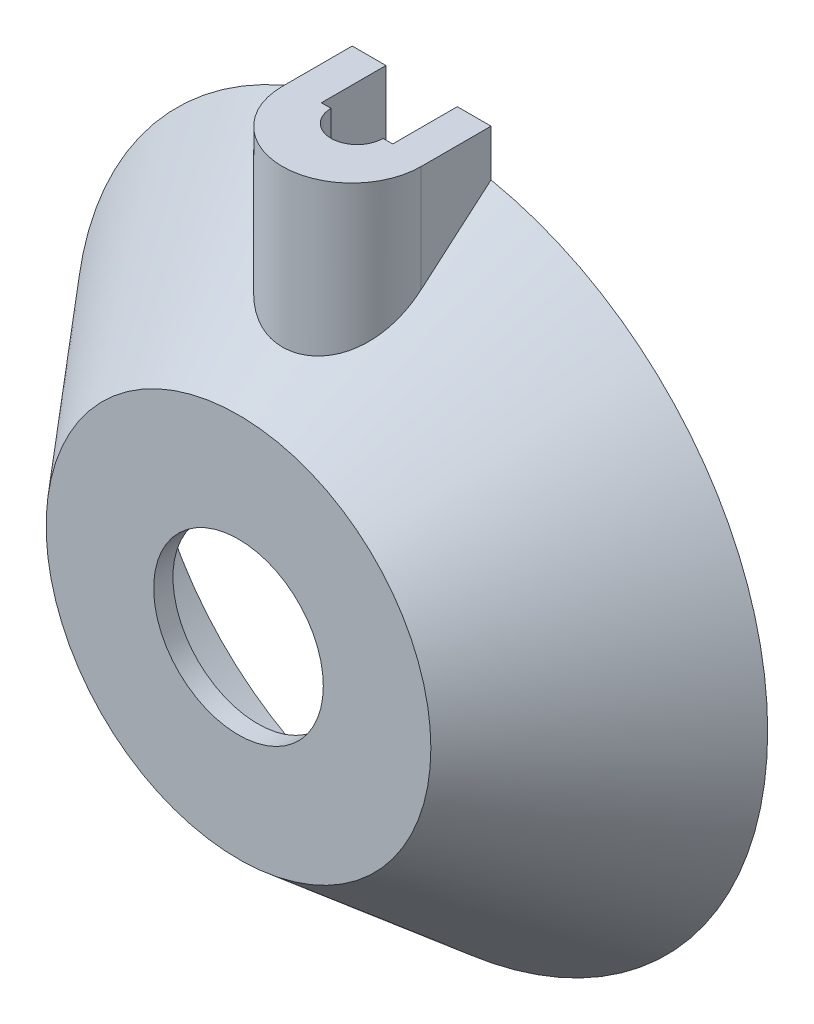
from build123d import *

# Parameters (mm, degrees)
SKETCH_1_R           = 35.9
EXTRUDE_1_DEPTH      = 19
EXTRUDE_1_TAPER      = 40
EXTRUDE_2_DEPTH      = 40
EXTRUDE_3_REACH      = 59.007
SKETCH_8_R           = 31
SKETCH_8_R_2         = 29
SKETCH_9_R           = 8.8
CUT_EXTRUDE_1_DEPTH  = 2
CUT_EXTRUDE_2_DEPTH  = 16
EXTRUDE_4_REACH      = 88.085
EXTRUDE_4_END_RADIUS = 31
SKETCH_11_W          = 2.2
SKETCH_11_H          = 6.7


with BuildPart() as part:
    # 草图1 → 凸台-拉伸1 (new body)
    with BuildSketch(Plane.XY):
        Circle(SKETCH_1_R)
    extrude(amount=EXTRUDE_1_DEPTH, taper=EXTRUDE_1_TAPER)

    # 草图6 → 凸台-拉伸2 (add)
    with BuildSketch(Plane(origin=(0, 0, 0), x_dir=(1, 0, 0), z_dir=(0, 1, 0))):
        with BuildLine():
            Line((-7.2, 0), (-7.2, -7.25))
            ThreePointArc((-7.2, -7.25), (0, -14.45), (7.2, -7.25))
            Line((7.2, -7.25), (7.2, 0))
            Line((7.2, 0), (-7.2, 0))
        make_face()
    extrude(amount=EXTRUDE_2_DEPTH)

    # 草图7 → 切除-旋转1 (revolve, cut)
    with BuildSketch(Plane(origin=(0, 0, 0), x_dir=(0, 0, -1), z_dir=(1, 0, 0)), mode=Mode.PRIVATE) as cut_revolve_1_sk:
        Polygon((-17, 0), (-17, -17.63530627), (0, -31.9), (0, 0), align=None)
    revolve(cut_revolve_1_sk.sketch.rotate(Axis((0, 0, -9.48864884), (0, 0, 1)), 270), axis=Axis((0, 0, -9.48864884), (0, 0, 1)), mode=Mode.SUBTRACT)

    # 凸台-拉伸3: up to this cone (the profile starts inside it)
    extrude_3_end = Plane(origin=(0, 0, 0), z_dir=(0, 0, -1)).offset(-38.016938604) * Cone(1e-06, 108.599579987, 129.423938604, align=(Align.CENTER, Align.CENTER, Align.MIN), mode=Mode.PRIVATE)
    # 草图8 → 凸台-拉伸3 (add, up to the surface)
    with BuildSketch(Plane(origin=(0, 0, 0), x_dir=(-1, 0, 0), z_dir=(0, 0, -1)), mode=Mode.PRIVATE) as extrude_3_sk1:
        Circle(SKETCH_8_R)
        Circle(SKETCH_8_R_2, mode=Mode.SUBTRACT)
    extrude_3_tool1 = extrude(extrude_3_sk1.sketch, amount=-EXTRUDE_3_REACH, mode=Mode.PRIVATE) & extrude_3_end
    add(extrude_3_tool1.solids().sort_by_distance((30.123188, 0, 0))[0])

    # 草图9 → 切除-拉伸1 (cut)
    with BuildSketch(Plane.XY.offset(19)):
        Circle(SKETCH_9_R)
    extrude(amount=-CUT_EXTRUDE_1_DEPTH, mode=Mode.SUBTRACT)

    # 草图10 → 切除-拉伸2 (cut)
    with BuildSketch(Plane(origin=(0, 40, 0), x_dir=(1, 0, 0), z_dir=(0, 1, 0))):
        with BuildLine():
            Line((3.7, 0), (3.7, -6.7))
            Line((3.7, -6.7), (2.7, -6.7))
            ThreePointArc((2.7, -6.7), (0, -9.4), (-2.7, -6.7))
            Line((-2.7, -6.7), (-3.7, -6.7))
            Line((-3.7, -6.7), (-3.7, 0))
            Line((-3.7, 0), (3.7, 0))
        make_face()
    extrude(amount=-CUT_EXTRUDE_2_DEPTH, mode=Mode.SUBTRACT)

    # 凸台-拉伸4: up to this cylinder (the profile starts outside it)
    extrude_4_end = Plane(origin=(0, 0, 3.35), z_dir=(0, 0, -1)) * Cylinder(EXTRUDE_4_END_RADIUS, 239.17, mode=Mode.PRIVATE)
    # 草图11 → 凸台-拉伸4 (add, up to the surface)
    with BuildSketch(Plane(origin=(0, 40, 0), x_dir=(1, 0, 0), z_dir=(0, 1, 0)), mode=Mode.PRIVATE) as extrude_4_sk1:
        with Locations((-4.8, -3.35)):
            Rectangle(SKETCH_11_W, SKETCH_11_H)
    extrude_4_tool1 = extrude(extrude_4_sk1.sketch, amount=-EXTRUDE_4_REACH, mode=Mode.PRIVATE) - extrude_4_end
    add(extrude_4_tool1.solids().sort_by_distance((-4.8, 40, 3.35))[0])
    # 草图11 → 凸台-拉伸4 (add, up to the surface)
    with BuildSketch(Plane(origin=(0, 40, 0), x_dir=(1, 0, 0), z_dir=(0, 1, 0)), mode=Mode.PRIVATE) as extrude_4_sk2:
        with Locations((4.8, -3.35)):
            Rectangle(SKETCH_11_W, SKETCH_11_H)
    extrude_4_tool2 = extrude(extrude_4_sk2.sketch, amount=-EXTRUDE_4_REACH, mode=Mode.PRIVATE) - extrude_4_end
    add(extrude_4_tool2.solids().sort_by_distance((4.8, 40, 3.35))[0])


solid = part.part
